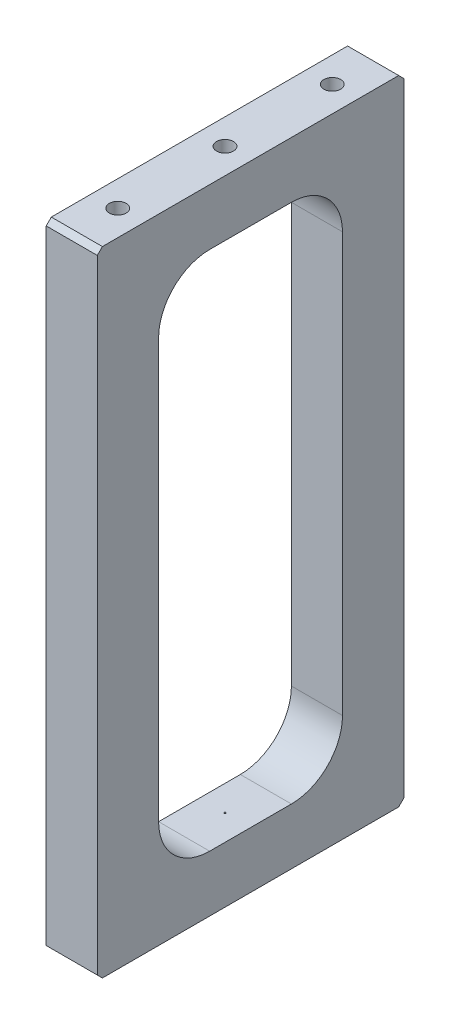
from build123d import *

# Parameters (mm, degrees)
SKETCH1_W             = 60
SKETCH1_H             = 124
BOSS_EXTRUDE1_DEPTH   = 5
SKETCH2_W             = 36
SKETCH2_H             = 102
CUT_EXTRUDE1_DEPTH    = 70.598850565
M4_TAPPED_HOLE1_D     = 3.3
M4_TAPPED_HOLE1_DEPTH = 10.1
M4_TAPPED_HOLE1_TIP   = 0.991420021
FILLET1_R             = 10
M4_TAPPED_HOLE2_D     = 3.3
M4_TAPPED_HOLE2_DEPTH = 10.1
M4_TAPPED_HOLE2_TIP   = 0.991420021
CHAMFER1_SIZE         = 1


with BuildPart() as part:
    # Sketch1 → Boss-Extrude1 (new, symmetric)
    with BuildSketch(Plane(origin=(0, 0, 0), x_dir=(0, 0, -1), z_dir=(1, 0, 0))):
        Rectangle(SKETCH1_W, SKETCH1_H)
    extrude(amount=BOSS_EXTRUDE1_DEPTH, both=True)

    # Sketch2 → Cut-Extrude1 (cut, through all)
    with BuildSketch(Plane(origin=(5, 0, 0), x_dir=(0, 0, -1), z_dir=(1, 0, 0))):
        Rectangle(SKETCH2_W, SKETCH2_H)
    extrude(amount=-CUT_EXTRUDE1_DEPTH, mode=Mode.SUBTRACT)

    # M4 Tapped Hole1
    with Locations(Plane(origin=(0, 62, 0), x_dir=(1, 0, 0), z_dir=(0, 1, 0))):
        with Locations((0, 0), (0, 21), (0, -21)):
            Hole(M4_TAPPED_HOLE1_D / 2, depth=M4_TAPPED_HOLE1_DEPTH)
            with Locations((0, 0, -(M4_TAPPED_HOLE1_DEPTH + M4_TAPPED_HOLE1_TIP / 2))):  # 118° drill point
                Cone(0, M4_TAPPED_HOLE1_D / 2, M4_TAPPED_HOLE1_TIP, mode=Mode.SUBTRACT)

    # Fillet1
    fillet1_edges = [part.edges().sort_by_distance(p)[0] for p in [
        (0, 51, -18),
        (0, -51, -18),
        (0, -51, 18),
        (0, 51, 18),
    ]]
    fillet(fillet1_edges, radius=FILLET1_R)

    # M4 Tapped Hole2
    with Locations(Plane(origin=(0, -62, 0), x_dir=(-1, 0, 0), z_dir=(0, -1, 0))):
        with Locations((0, 0), (0, 21), (0, -21)):
            Hole(M4_TAPPED_HOLE2_D / 2, depth=M4_TAPPED_HOLE2_DEPTH)
            with Locations((0, 0, -(M4_TAPPED_HOLE2_DEPTH + M4_TAPPED_HOLE2_TIP / 2))):  # 118° drill point
                Cone(0, M4_TAPPED_HOLE2_D / 2, M4_TAPPED_HOLE2_TIP, mode=Mode.SUBTRACT)

    # Chamfer1
    chamfer1_edges = [part.edges().sort_by_distance(p)[0] for p in [
        (0, -62, -30),
        (0, -62, 30),
        (0, 62, 30),
        (0, 62, -30),
    ]]
    chamfer(chamfer1_edges, length=CHAMFER1_SIZE)


solid = part.part
